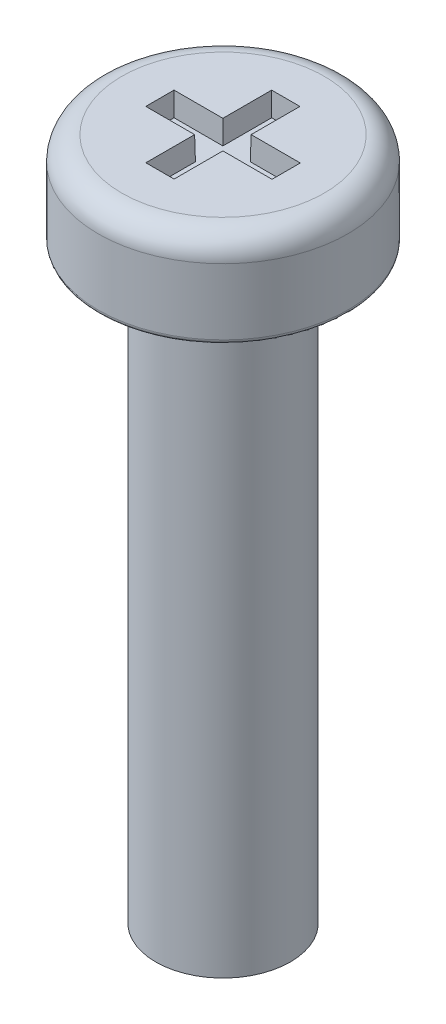
from build123d import *

# Parameters (mm, degrees)
SKETCH1_R           = 2.65
BOSS_EXTRUDE1_DEPTH = 2
SKETCH2_R           = 1.43
BOSS_EXTRUDE2_DEPTH = 12.5
FILLET1_R           = 0.5
FILLET2_R           = 0.1
CUT_EXTRUDE1_DEPTH  = 0.5
CUT_EXTRUDE1_DRAFT  = -1


with BuildPart() as part:
    # Sketch1 → Boss-Extrude1 (new body)
    with BuildSketch(Plane(origin=(0, 0, 0), x_dir=(1, 0, 0), z_dir=(0, 1, 0))):
        with Locations(Location((0, 0, 0), (0, 0, 270))):
            Circle(SKETCH1_R)
    extrude(amount=BOSS_EXTRUDE1_DEPTH)

    # Sketch2 → Boss-Extrude2 (add)
    with BuildSketch(Plane.XZ):
        with Locations(Location((0, 0, 0), (0, 0, 90))):
            Circle(SKETCH2_R)
    extrude(amount=BOSS_EXTRUDE2_DEPTH)

    # Fillet1
    fillet1_edges = [part.edges().sort_by_distance(p)[0] for p in [
        (0, 2, -2.65),
    ]]
    fillet(fillet1_edges, radius=FILLET1_R)

    # Fillet2
    fillet2_edges = [part.edges().sort_by_distance(p)[0] for p in [
        (0, 0, -2.65),
    ]]
    fillet(fillet2_edges, radius=FILLET2_R)


with BuildPart() as cut_extrude1_tool:
    # Sketch3 → Cut-Extrude1 (with draft: the straight prism first)
    with BuildSketch(Plane(origin=(0, 2, 0), x_dir=(1, 0, 0), z_dir=(0, 1, 0))):
        Polygon((0.296573117, 0.3), (0.296573117, 1.336133674), (-0.303426883, 1.336133674), (-0.303426883, 0.3), (-1.340662941, 0.3), (-1.340662941, -0.3), (-0.303426883, -0.3), (-0.303426883, -1.336133674), (0.296573117, -1.336133674), (0.296573117, -0.3), (1.340662941, -0.3), (1.340662941, 0.3), align=None)
    extrude(amount=-CUT_EXTRUDE1_DEPTH)
    # Cut-Extrude1: the draft: its side faces are tilted about the plane it starts from
    cut_extrude1_sides = [cut_extrude1_tool.faces().sort_by_distance(p)[0] for p in [
        (0.296573117, 1.75, -0.818066837),
        (-0.003426883, 1.75, -1.336133674),
        (-0.303426883, 1.75, -0.818066837),
        (-0.822044912, 1.75, -0.3),
        (-1.340662941, 1.75, 0),
        (-0.822044912, 1.75, 0.3),
        (-0.303426883, 1.75, 0.818066837),
        (-0.003426883, 1.75, 1.336133674),
        (0.296573117, 1.75, 0.818066837),
        (0.818618029, 1.75, 0.3),
        (1.340662941, 1.75, 0),
        (0.818618029, 1.75, -0.3),
    ]]
    draft(cut_extrude1_sides, Plane(origin=(0, 2, 0), x_dir=(1, 0, 0), z_dir=(0, 1, 0)), CUT_EXTRUDE1_DRAFT)


with BuildPart() as part_1:
    add(part.part)

    # Cut-Extrude1: cut by cut_extrude1_tool
    add(cut_extrude1_tool.part, mode=Mode.SUBTRACT)


solid = part_1.part
